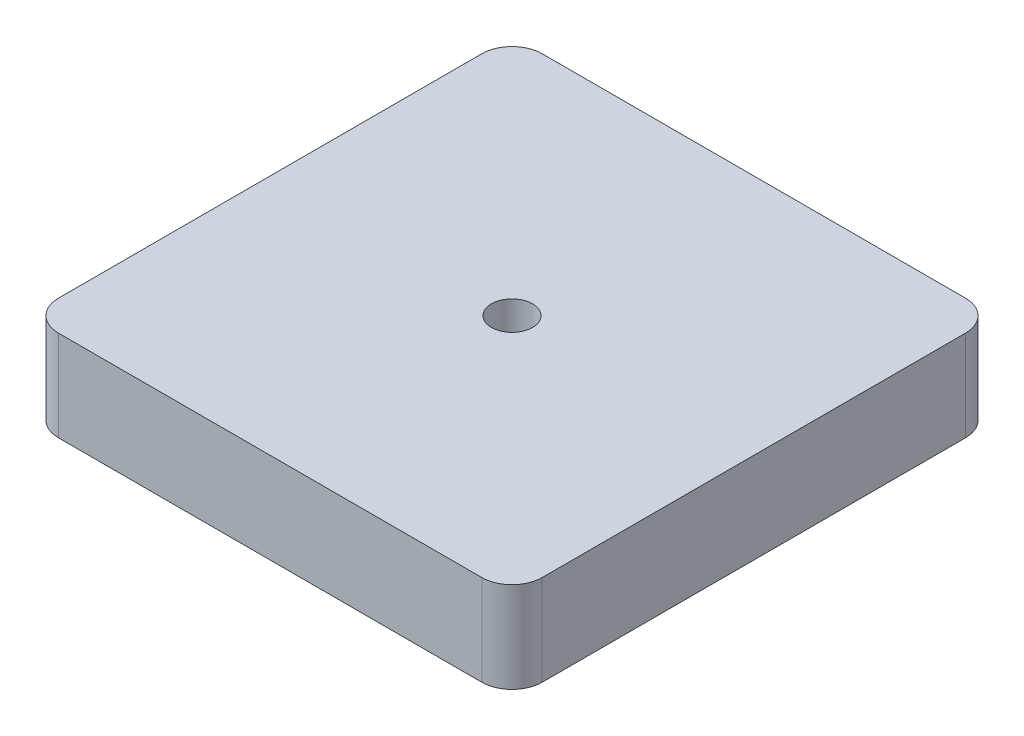
SolidWorks part; units mm, degrees
ref_plane "前视基准面" through (0, 0, 0) normal (0, 0, 1) x (1, 0, 0)
ref_plane "上视基准面" through (0, 0, 0) normal (0, 1, 0) x (1, 0, 0)
ref_plane "右视基准面" through (0, 0, 0) normal (1, 0, 0) x (0, 0, -1)
sketch "草图1" plane through (0, 0, 0) normal (0, 1, 0) x (1, 0, 0)
  line L1 (-40, 40) -> (40, 40)
  line L2 (-40, 40) -> (-40, -40)
  line L3 (-40, -40) -> (40, -40)
  line L4 (40, 40) -> (40, -40)
  line L5 (-40, 40) -> (40, -40) construction
  line L6 (-40, -40) -> (40, 40) construction
  point P0 (0, 0)
  dimension "D1" = 80
  dimension "D2" = 80
extrude "凸台-拉伸1" add sketch "草图1" along normal blind 15
fillet "圆角1" radius 5 4 edges at (-40, 7.5, 40) (40, 7.5, 40) (40, 7.5, -40) (-40, 7.5, -40)
hole_wizard "M8 螺纹孔1" positions "草图4" profile "草图5" tap size "M8" standard "GB"
sketch "草图4" plane through (0, 0, 0) normal (0, -1, 0) x (-1, 0, 0)
  point P0 (0, 0)
sketch "草图5" plane through (0, 0, 0) normal (1, 0, 0) x (0, 0, -1)
  line L0 (0, 0) -> (0, 21.7929)
  line L1 (0, 21.7929) -> (3.4, 19.75)
  line L2 (3.4, 19.75) -> (3.4, 0)
  line L5 (3.4, 0) -> (0, 0)
  line L10 (0, 21.7929) -> (-3.4, 19.75) construction
  line L11 (0, -6.35) -> (0, 107.95) construction
  dimension "螺纹孔钻头直径" = 6.8
  dimension "螺纹孔钻头深度" = 19.75
  dimension "导头角度" = 118
cosmetic thread "孔螺蚊线1" parameters "D1"=15, "D2"=8
